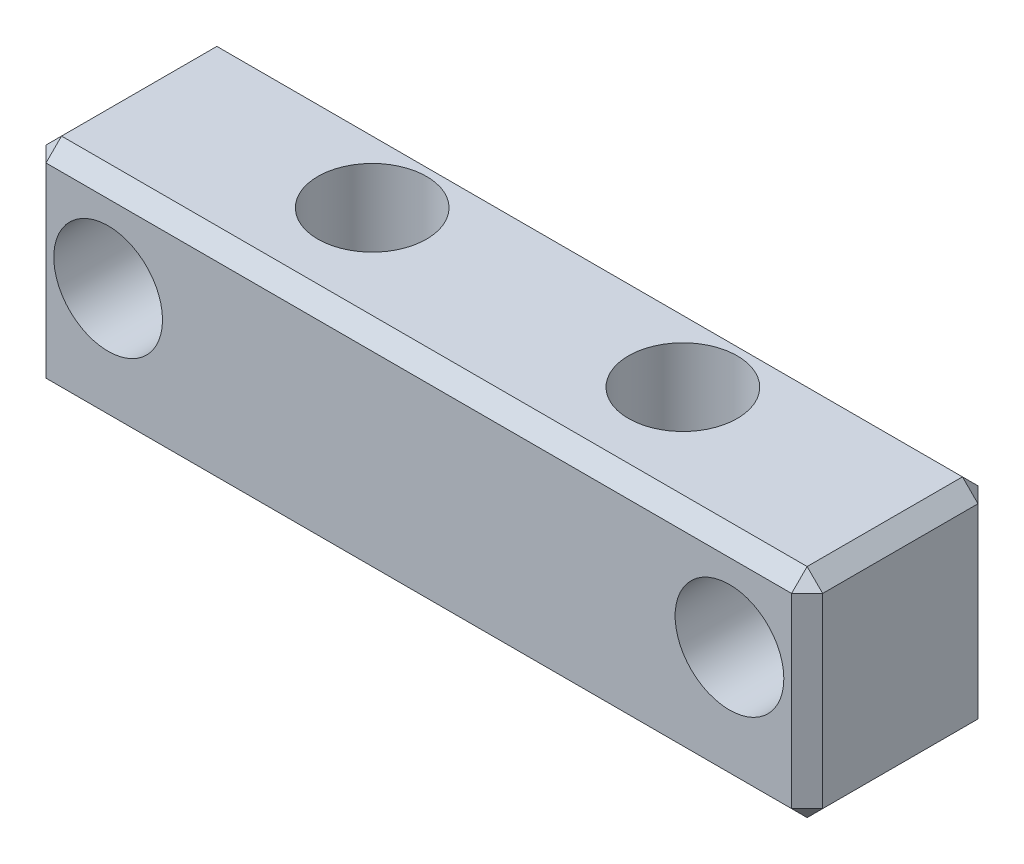
from build123d import *

# Parameters (mm, degrees)
SKETCH1_W                      = 25
SKETCH1_H                      = 7
BOSS_EXTRUDE1_DEPTH            = 6
F_3_5_3_5_DIAMETER_HOLE2_D     = 3.5
F_3_5_3_5_DIAMETER_HOLE3_D     = 3.5
F_3_5_3_5_DIAMETER_HOLE3_DEPTH = 3
F_3_5_3_5_DIAMETER_HOLE3_TIP   = 1.051506083
CHAMFER1_SIZE                  = 0.5


with BuildPart() as part:
    # Sketch1 → Boss-Extrude1 (new body)
    with BuildSketch(Plane.XY):
        Rectangle(SKETCH1_W, SKETCH1_H)
    extrude(amount=BOSS_EXTRUDE1_DEPTH)

    # Ø3.5 (3.5) Diameter Hole2 (through all)
    with Locations(Plane.XY.offset(6)):
        with Locations((-10, 0.5), (10, 0.5)):
            Hole(F_3_5_3_5_DIAMETER_HOLE2_D / 2)

    # Ø3.5 (3.5) Diameter Hole3
    with Locations(Plane(origin=(0, 3.5, 0), x_dir=(1, 0, 0), z_dir=(0, 1, 0))):
        with Locations((5, -2.5), (-5, -2.5)):
            Hole(F_3_5_3_5_DIAMETER_HOLE3_D / 2, depth=F_3_5_3_5_DIAMETER_HOLE3_DEPTH)
            with Locations((0, 0, -(F_3_5_3_5_DIAMETER_HOLE3_DEPTH + F_3_5_3_5_DIAMETER_HOLE3_TIP / 2))):  # 118° drill point
                Cone(0, F_3_5_3_5_DIAMETER_HOLE3_D / 2, F_3_5_3_5_DIAMETER_HOLE3_TIP, mode=Mode.SUBTRACT)

    # Chamfer1
    chamfer1_edges = [part.edges().sort_by_distance(p)[0] for p in [
        (-12.5, 0, 6),
        (0, -3.5, 6),
        (12.5, 0, 6),
        (0, -3.5, 0),
        (-12.5, 0, 0),
        (0, 3.5, 0),
        (12.5, 0, 0),
        (0, 3.5, 6),
        (12.5, -3.5, 3),
        (-12.5, -3.5, 3),
        (-12.5, 3.5, 3),
        (12.5, 3.5, 3),
    ]]
    chamfer(chamfer1_edges, length=CHAMFER1_SIZE)


solid = part.part
